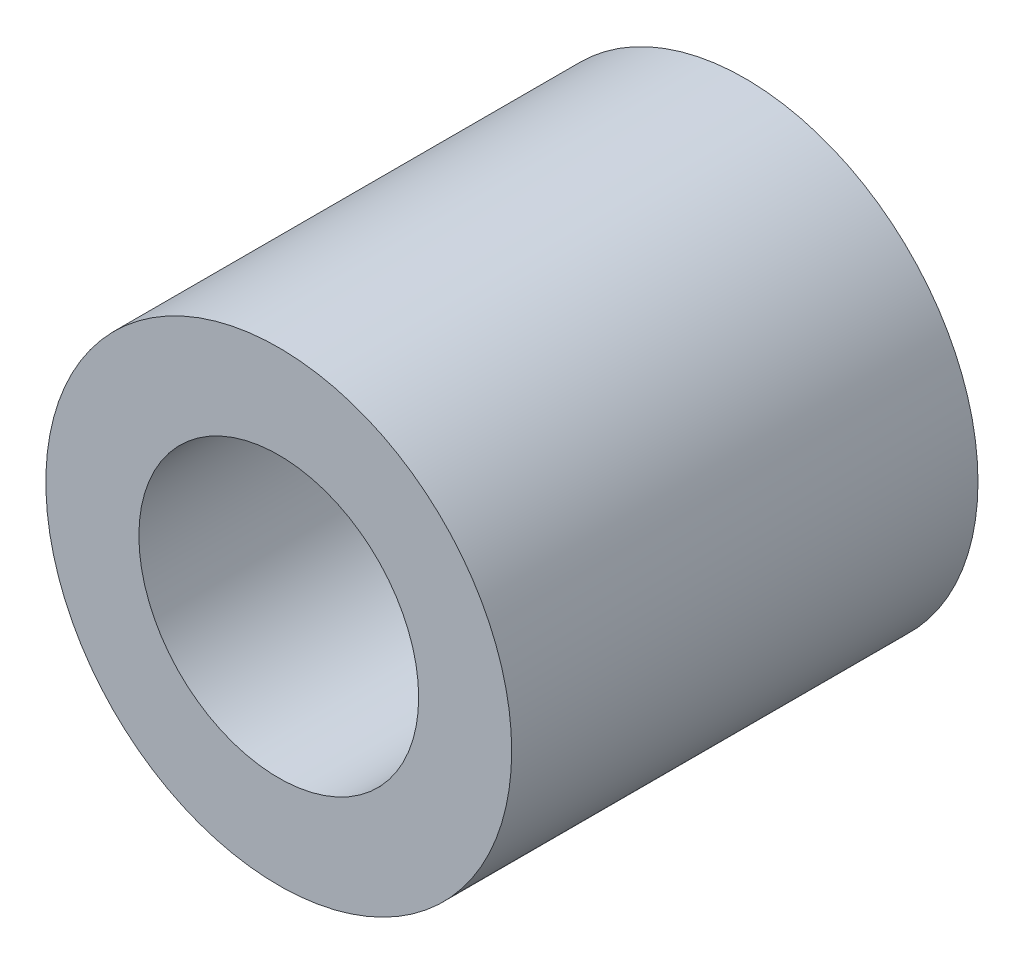
SolidWorks part; units mm, degrees
ref_plane "Front Plane" through (0, 0, 0) normal (0, 0, 1) x (1, 0, 0)
ref_plane "Top Plane" through (0, 0, 0) normal (0, 1, 0) x (1, 0, 0)
ref_plane "Right Plane" through (0, 0, 0) normal (1, 0, 0) x (0, 0, -1)
other "Configuration Table"
sketch "Sketch1" plane through (0, 0, 0) normal (0, 0, 1) x (1, 0, 0)
  circle A0 centre (0, 0) radius 4.995
  circle A1 centre (0, 0) radius 3
  dimension "D1" = 6
  dimension "D2" = 9.99
extrude "Boss-Extrude1" add sketch "Sketch1" along normal blind 10
